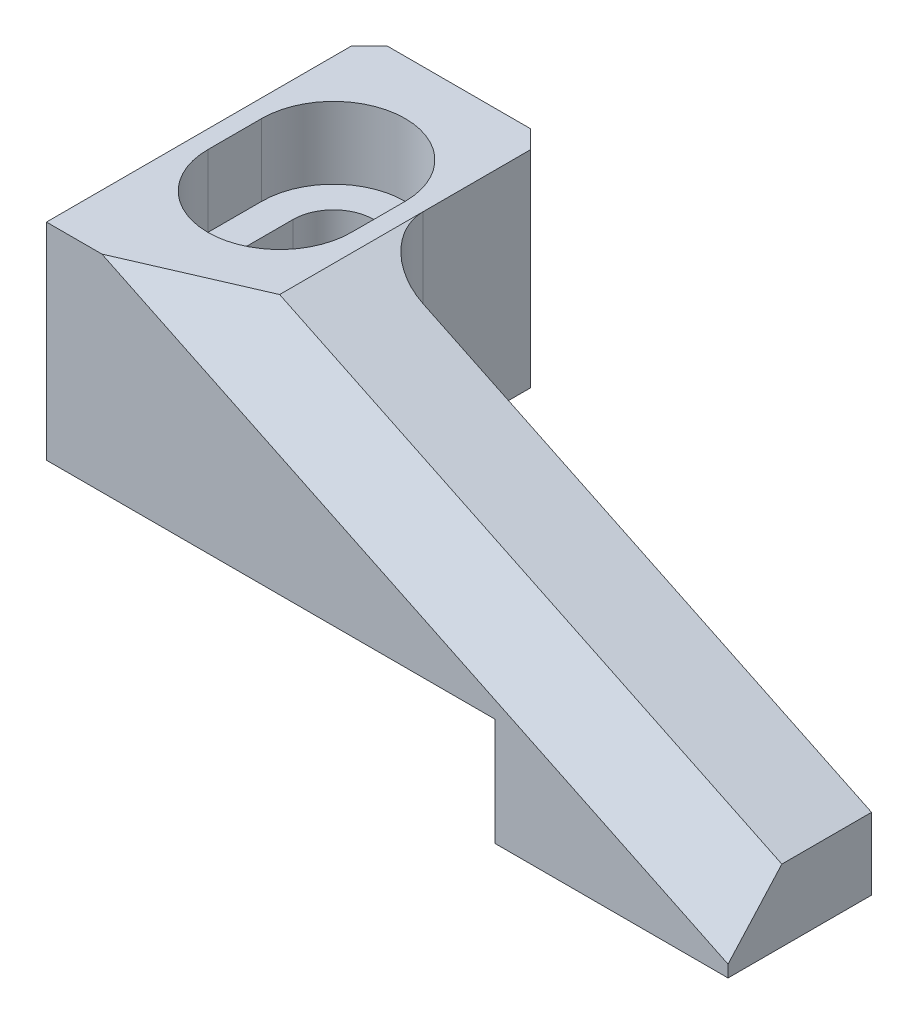
from build123d import *

# Parameters (mm, degrees)
BOSS_EXTRUDE1_DEPTH = 18
CHAMFER1_SIZE       = 3
CUT_EXTRUDE1_DEPTH  = 20
CUT_EXTRUDE3_DEPTH  = 4
SKETCH3_W           = 25
SKETCH3_H           = 6
CUT_EXTRUDE2_DEPTH  = 46.543934832
SKETCH5_W           = 28
SKETCH5_H           = 10
CUT_EXTRUDE4_DEPTH  = 46.543934832
FILLET1_R           = 3
CHAMFER2_SIZE       = 1


with BuildPart() as part:
    # Sketch1 → Boss-Extrude1 (new body)
    with BuildSketch(Plane.XY):
        Polygon((0, 17.5), (0, 0), (38, 0), (38, 4), (10, 17.5), align=None)
    extrude(amount=BOSS_EXTRUDE1_DEPTH)

    # Chamfer1
    chamfer1_edges = [part.edges().sort_by_distance(p)[0] for p in [
        (24, 10.75, 18),
    ]]
    chamfer(chamfer1_edges, length=CHAMFER1_SIZE)

    # Sketch2 → Cut-Extrude1 (cut)
    with BuildSketch(Plane(origin=(0, 17.5, 0), x_dir=(1, 0, 0), z_dir=(0, 1, 0))):
        with BuildLine():
            Line((2.75, -10), (2.75, -7))
            ThreePointArc((2.75, -7), (5, -4.75), (7.25, -7))
            Line((7.25, -7), (7.25, -10))
            ThreePointArc((7.25, -10), (5, -12.25), (2.75, -10))
        make_face()
    extrude(amount=-CUT_EXTRUDE1_DEPTH, mode=Mode.SUBTRACT)

    # Sketch4 → Cut-Extrude3 (cut)
    with BuildSketch(Plane(origin=(0, 17.5, 0), x_dir=(1, 0, 0), z_dir=(0, 1, 0))):
        with BuildLine():
            Line((9, -7), (9, -10))
            ThreePointArc((9, -10), (5, -14), (1, -10))
            Line((1, -10), (1, -7))
            ThreePointArc((1, -7), (5, -3), (9, -7))
        make_face()
    extrude(amount=-CUT_EXTRUDE3_DEPTH, mode=Mode.SUBTRACT)

    # Sketch3 → Cut-Extrude2 (cut, through all)
    with BuildSketch(Plane.XY.offset(18)):
        with Locations((12.5, 3)):
            Rectangle(SKETCH3_W, SKETCH3_H)
    extrude(amount=-CUT_EXTRUDE2_DEPTH, mode=Mode.SUBTRACT)

    # Sketch5 → Cut-Extrude4 (cut, through all)
    with BuildSketch(Plane(origin=(0, 17.5, 0), x_dir=(-1, 0, 0), z_dir=(0, 1, 0))):
        with Locations((-24, 5)):
            Rectangle(SKETCH5_W, SKETCH5_H)
    extrude(amount=-CUT_EXTRUDE4_DEPTH, mode=Mode.SUBTRACT)

    # Fillet1
    fillet1_edges = [part.edges().sort_by_distance(p)[0] for p in [
        (10, 11.75, 10),
    ]]
    fillet(fillet1_edges, radius=FILLET1_R)

    # Chamfer2
    chamfer2_edges = [part.edges().sort_by_distance(p)[0] for p in [
        (0, 11.75, 0),
        (10, 11.75, 0),
    ]]
    chamfer(chamfer2_edges, length=CHAMFER2_SIZE)


solid = part.part
